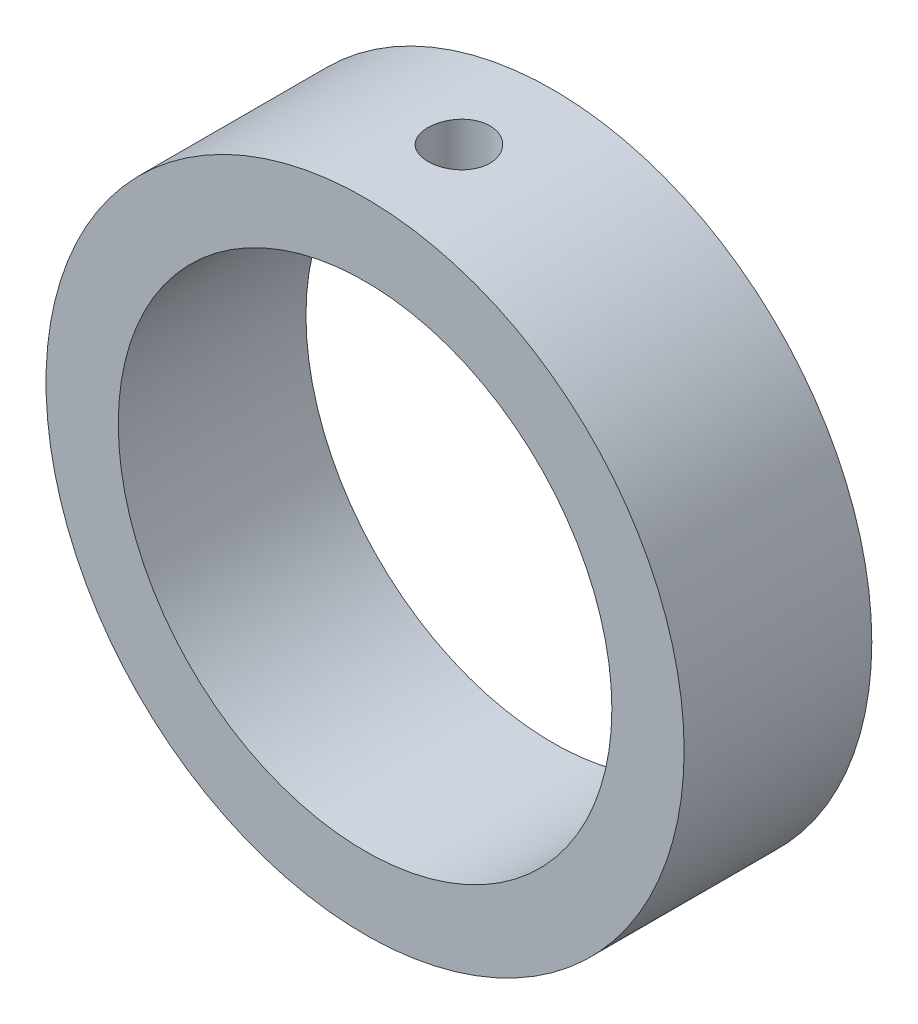
from build123d import *

# Parameters (mm, degrees)
SKETCH_1_R      = 17
SKETCH_1_R_2    = 13.15
EXTRUDE_1_DEPTH = 5
SKETCH_8_W      = 1.65
SKETCH_8_H      = 17


with BuildPart() as part:
    # 草图1 → 凸台-拉伸1 (new, symmetric)
    with BuildSketch(Plane.XY):
        Circle(SKETCH_1_R)
        Circle(SKETCH_1_R_2, mode=Mode.SUBTRACT)
    extrude(amount=EXTRUDE_1_DEPTH, both=True)

    # 草图8 → M4 螺纹孔2 (revolve, cut)
    with BuildSketch(Plane(origin=(0, 0, 0), x_dir=(0, 0, -1), z_dir=(1, 0, 0))):
        with Locations((0.825, 8.5)):
            Rectangle(SKETCH_8_W, SKETCH_8_H)
    revolve(axis=Axis((0, -6.35, 0), (0, 1, 0)), mode=Mode.SUBTRACT)


solid = part.part
